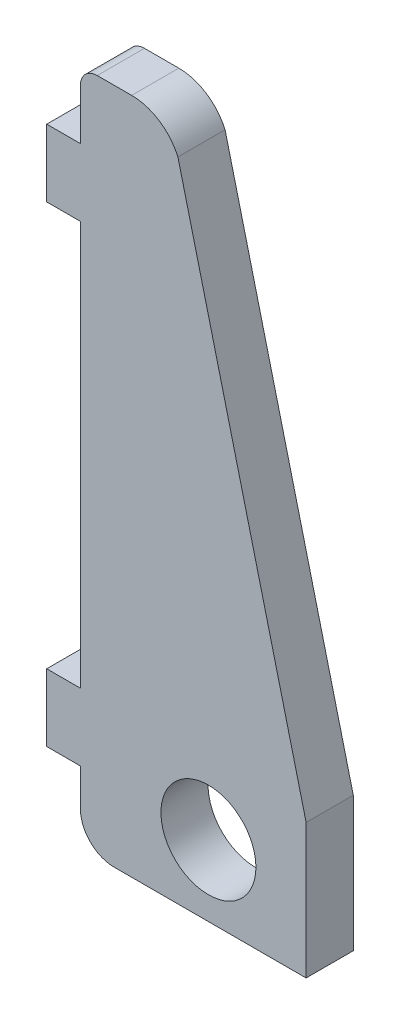
SolidWorks part; units mm, degrees
material "Q235"
ref_plane "Front Plane" through (0, 0, 0) normal (0, 0, 1) x (1, 0, 0)
ref_plane "Top Plane" through (0, 0, 0) normal (0, 1, 0) x (1, 0, 0)
ref_plane "Right Plane" through (0, 0, 0) normal (1, 0, 0) x (0, 0, -1)
sketch "Sketch2" plane through (0, 0, 0) normal (0, 0, 1) x (1, 0, 0)
  line L0 (10, 181) -> (10, 196)
  line L1 (15, 201) -> (25.2095, 201)
  line L2 (10, 10) -> (10, 21)
  line L3 (10, 21) -> (0, 21)
  line L4 (0, 21) -> (0, 41)
  line L5 (0, 41) -> (10, 41)
  line L6 (10, 181) -> (0, 181)
  line L7 (0, 181) -> (0, 161)
  line L8 (0, 161) -> (10, 161)
  line L9 (10, 161) -> (10, 101)
  line L10 (76.9975, 0) -> (76.9975, 10)
  line L11 (10, 101) -> (10, 41)
  line L12 (76.9975, 10) -> (76.9975, 30)
  line L13 (76.9975, 30) -> (76.9975, 40)
  line L14 (20, 0) -> (76.9975, 0)
  line L15 (76.9975, 40) -> (38.9408, 192.0376)
  arc A0 (10, 10) -> (20, 0) centre (20, 10) ccw
  arc A1 (15, 201) -> (10, 196) centre (15, 196) ccw
  arc A2 (38.9408, 192.0376) -> (25.2095, 201) centre (25.2095, 186) ccw
  circle A3 centre (48, 21) radius 14.1
extrude "Boss-Extrude2" add sketch "Sketch2" along normal blind 14
equation "\"图号代码1\"= \"图号代码\""
equation "\"名称代码2\"= \"名称代码\""
